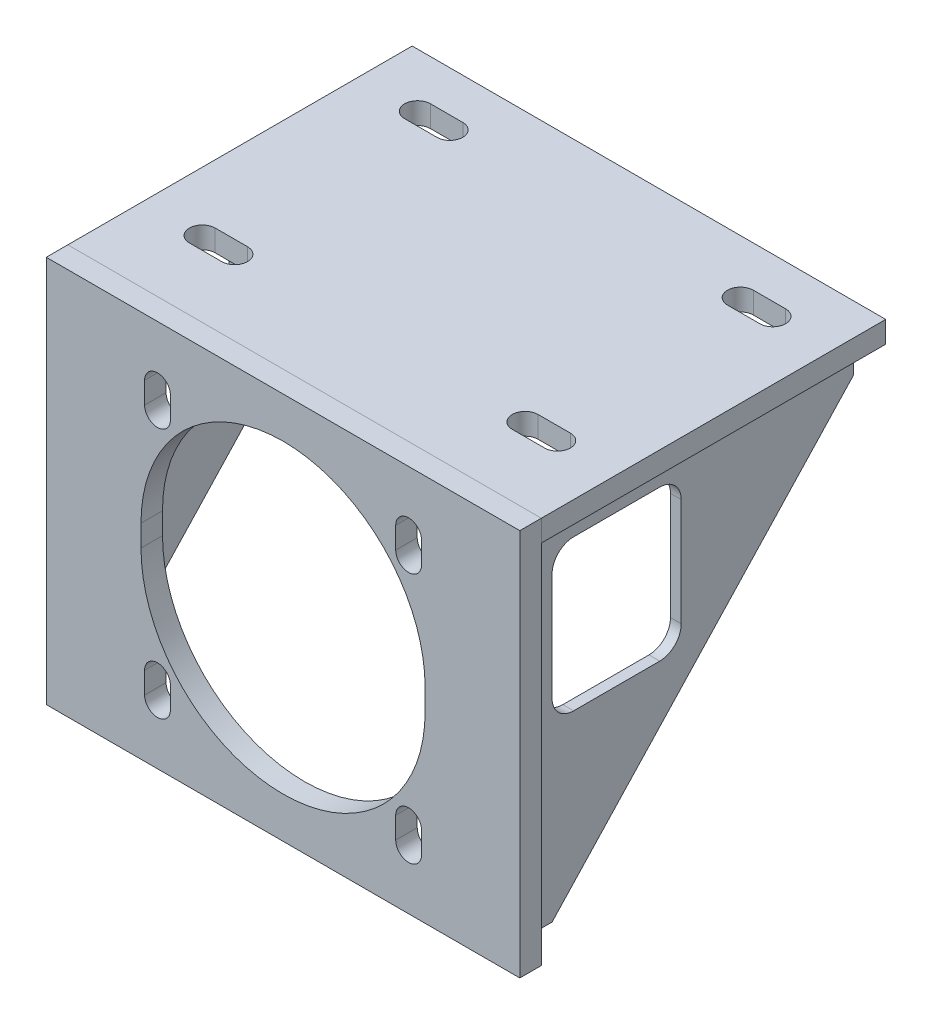
from build123d import *

# Parameters (mm, degrees)
SKETCH1_W            = 220
SKETCH1_H            = 180
BOSS_EXTRUDE1_DEPTH  = 5
SKETCH2_R            = 65.5
CUT_EXTRUDE1_DEPTH   = 55
SKETCH3_R            = 5.5
CUT_EXTRUDE2_DEPTH   = 55
CIRPATTERN1_COUNT    = 4
SKETCH4_W            = 220
SKETCH4_H            = 10
BOSS_EXTRUDE2_DEPTH  = 160
BOSS_EXTRUDE3_START  = -5
BOSS_EXTRUDE3_DEPTH  = 5
CUT_EXTRUDE3_DEPTH   = 15
CUT_EXTRUDE4_DEPTH   = 16
CUT_EXTRUDE5_DEPTH   = 16
LPATTERN1_COUNT      = 2
LPATTERN1_PITCH      = 150
LPATTERN1_COUNT_DIR2 = 2
LPATTERN1_PITCH_DIR2 = 100
CUT_EXTRUDE6_DEPTH   = 317


with BuildPart() as part:
    # Sketch1 → Boss-Extrude1 (new, symmetric)
    with BuildSketch(Plane.XY):
        Rectangle(SKETCH1_W, SKETCH1_H)
    extrude(amount=BOSS_EXTRUDE1_DEPTH, both=True)

    # Sketch2 → Cut-Extrude1 (cut)
    with BuildSketch(Plane(origin=(0, 0, -5), x_dir=(-1, 0, 0), z_dir=(0, 0, -1))):
        Circle(SKETCH2_R)
    extrude(amount=-CUT_EXTRUDE1_DEPTH, mode=Mode.SUBTRACT)

    # Sketch3 → Cut-Extrude2 (cut)
    with BuildSketch(Plane(origin=(0, 0, -5), x_dir=(-1, 0, 0), z_dir=(0, 0, -1))):
        with Locations((-58.336309448, 58.336309448)):
            Circle(SKETCH3_R)
    cut_extrude2 = extrude(amount=-CUT_EXTRUDE2_DEPTH, mode=Mode.SUBTRACT)

    # CirPattern1: Cut-Extrude2 ×4 about axis
    cirpattern1_axis = Axis((0, 0, 0), (0, 0, 1))
    for i in range(1, CIRPATTERN1_COUNT):
        add(cut_extrude2.rotate(cirpattern1_axis, i * 360 / CIRPATTERN1_COUNT), mode=Mode.SUBTRACT)

    # Sketch7 → Cut-Extrude3 (cut)
    with BuildSketch(Plane.XY.offset(5)):
        with BuildLine():
            Line((-52.336309448, 63.336309448), (-52.336309448, 53.336309448))
            ThreePointArc((-52.336309448, 53.336309448), (-58.336309448, 47.336309448), (-64.336309448, 53.336309448))
            Line((-64.336309448, 53.336309448), (-64.336309448, 63.336309448))
            ThreePointArc((-64.336309448, 63.336309448), (-58.336309448, 69.336309448), (-52.336309448, 63.336309448))
        make_face()
        with BuildLine():
            Line((64.336309448, 63.336309448), (64.336309448, 53.336309448))
            ThreePointArc((64.336309448, 53.336309448), (58.336309448, 47.336309448), (52.336309448, 53.336309448))
            Line((52.336309448, 53.336309448), (52.336309448, 63.336309448))
            ThreePointArc((52.336309448, 63.336309448), (58.336309448, 69.336309448), (64.336309448, 63.336309448))
        make_face()
        with BuildLine():
            Line((52.336309448, -63.336309448), (52.336309448, -53.336309448))
            ThreePointArc((52.336309448, -53.336309448), (58.336309448, -47.336309448), (64.336309448, -53.336309448))
            Line((64.336309448, -53.336309448), (64.336309448, -63.336309448))
            ThreePointArc((64.336309448, -63.336309448), (58.336309448, -69.336309448), (52.336309448, -63.336309448))
        make_face()
        with BuildLine():
            Line((-52.336309448, -53.336309448), (-52.336309448, -63.336309448))
            ThreePointArc((-52.336309448, -63.336309448), (-58.336309448, -69.336309448), (-64.336309448, -63.336309448))
            Line((-64.336309448, -63.336309448), (-64.336309448, -53.336309448))
            ThreePointArc((-64.336309448, -53.336309448), (-58.336309448, -47.336309448), (-52.336309448, -53.336309448))
        make_face()
    extrude(amount=-CUT_EXTRUDE3_DEPTH, mode=Mode.SUBTRACT)

    # Sketch8 → Cut-Extrude4 (cut)
    with BuildSketch(Plane.XY.offset(5)):
        with BuildLine():
            Line((66, 5), (66, -5))
            ThreePointArc((66, -5), (0, -71), (-66, -5))
            Line((-66, -5), (-66, 5))
            ThreePointArc((-66, 5), (0, 71), (66, 5))
        make_face()
    extrude(amount=-CUT_EXTRUDE4_DEPTH, mode=Mode.SUBTRACT)


with BuildPart() as body_2:
    # Sketch4 → Boss-Extrude2 (new body)
    with BuildSketch(Plane(origin=(0, 0, -5), x_dir=(-1, 0, 0), z_dir=(0, 0, -1))):
        with Locations((0, 85)):
            Rectangle(SKETCH4_W, SKETCH4_H)
    extrude(amount=BOSS_EXTRUDE2_DEPTH)

    # Sketch9 → Cut-Extrude5 (cut)
    with BuildSketch(Plane.XZ.offset(-80)):
        with BuildLine():
            Line((67.5, -34), (82.5, -34))
            ThreePointArc((82.5, -34), (88.5, -40), (82.5, -46))
            Line((82.5, -46), (67.5, -46))
            ThreePointArc((67.5, -46), (61.5, -40), (67.5, -34))
        make_face()
    cut_extrude5 = extrude(amount=-CUT_EXTRUDE5_DEPTH, mode=Mode.SUBTRACT)

    # LPattern1: Cut-Extrude5 2 × 2
    with Locations(*[(-i * LPATTERN1_PITCH, 0, -j * LPATTERN1_PITCH_DIR2) for i in range(LPATTERN1_COUNT) for j in range(LPATTERN1_COUNT_DIR2) if (i, j) != (0, 0)]):
        add(cut_extrude5, mode=Mode.SUBTRACT)


with BuildPart() as body_3:
    # Sketch6 → Boss-Extrude3 (new body)
    with BuildSketch(Plane.ZY.offset(110).offset(BOSS_EXTRUDE3_START)):
        Polygon((-5, 70), (-5, -80), (-15, -80), (-155, 70), (-155, 80), (-15, 80), align=None)
    extrude(amount=-BOSS_EXTRUDE3_DEPTH)


with BuildPart() as body_4:
    # Mirror1: mirrored copy
    add(body_3.part.mirror(Plane(origin=(0, 0, 0), x_dir=(0, 0, 1), z_dir=(1, 0, 0))))


with BuildPart() as cut_extrude6_tool:
    # Sketch10 → Cut-Extrude6 (new body)
    with BuildSketch(Plane.ZY.offset(105)):
        with BuildLine():
            Line((-65, 70), (-25, 70))
            ThreePointArc((-25, 70), (-17.928932188, 67.071067812), (-15, 60))
            Line((-15, 60), (-15, 10))
            ThreePointArc((-15, 10), (-17.928932188, 2.928932188), (-25, 0))
            Line((-25, 0), (-65, 0))
            ThreePointArc((-65, 0), (-72.071067812, 2.928932188), (-75, 10))
            Line((-75, 10), (-75, 60))
            ThreePointArc((-75, 60), (-72.071067812, 67.071067812), (-65, 70))
        make_face()
    extrude(amount=-CUT_EXTRUDE6_DEPTH)


with BuildPart() as body_3_1:
    add(body_3.part)

    # Cut-Extrude6: cut by cut_extrude6_tool
    add(cut_extrude6_tool.part, mode=Mode.SUBTRACT)


with BuildPart() as body_4_1:
    add(body_4.part)

    # Cut-Extrude6: cut by cut_extrude6_tool
    add(cut_extrude6_tool.part, mode=Mode.SUBTRACT)


solid = Compound([part.part, body_2.part, body_3_1.part, body_4_1.part])
